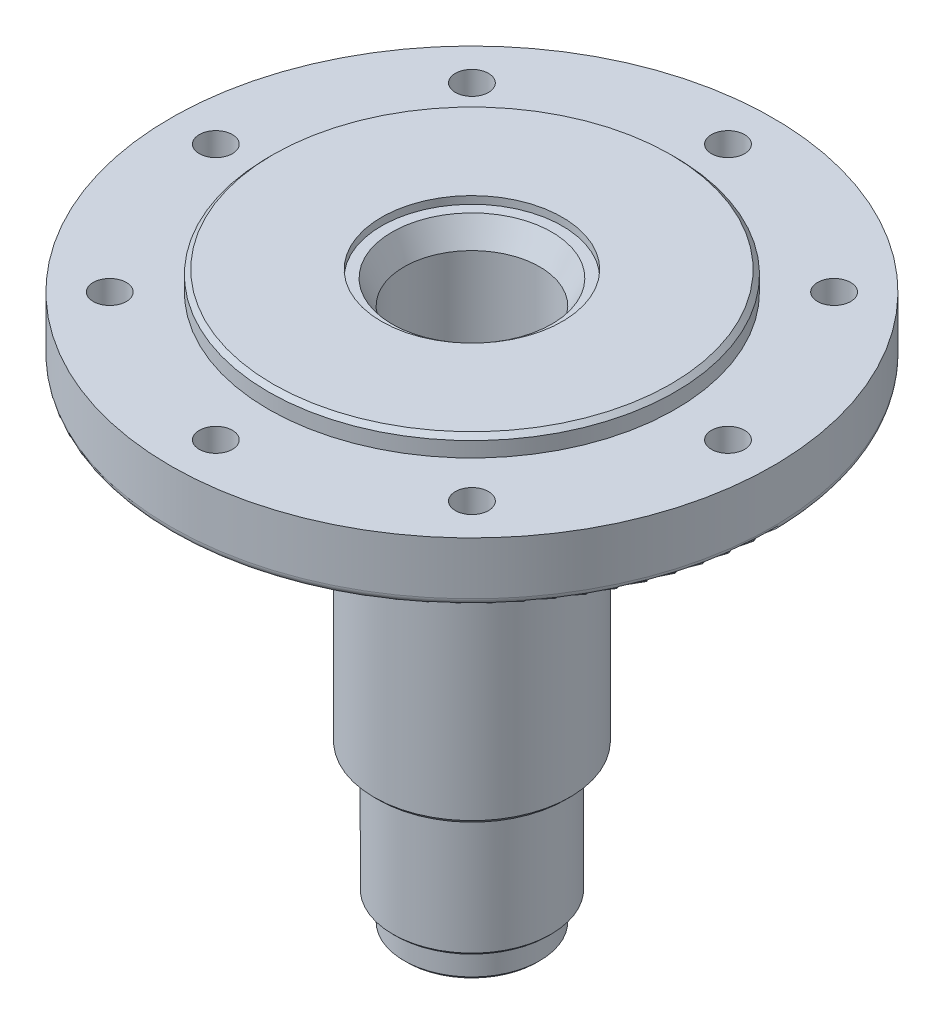
from build123d import *

# Parameters (mm, degrees)
SKETCH_2_R          = 20
CUT_EXTRUDE_1_DEPTH = 5
CUT_EXTRUDE_2_REACH = 424.606
SKETCH_3_R          = 11
SKETCH_5_R          = 120
SKETCH_5_R_2        = 80
CUT_EXTRUDE_3_DEPTH = 8
EXTRUDE_START       = 26
SKETCH_6_R          = 52.5
SKETCH_6_R_2        = 45
EXTRUDE_1_DEPTH     = 26
SKETCH_7_R          = 45
SKETCH_7_R_2        = 30
EXTRUDE_2_DEPTH     = 10
CHAMFER_1_SIZE      = 2
CHAMFER_2_SIZE      = 2


with BuildPart() as part:
    # 草图1 → 旋转1 (revolve)
    with BuildSketch(Plane.XY, mode=Mode.PRIVATE) as revolve_1_sk:
        with BuildLine():
            Line((60, 198.020625577), (132, 198.020625577))
            Line((132, 198.020625577), (135, 195.020625577))
            Line((135, 195.020625577), (135, 185.020625577))
            Line((135, 185.020625577), (200, 185.020625577))
            Line((200, 185.020625577), (200, 150.020625577))
            ThreePointArc((200, 150.020625577), (198.535533906, 146.485091671), (195, 145.020625577))
            Line((195, 145.020625577), (145, 145.020625577))
            Line((145, 145.020625577), (145, 140.020625577))
            Line((145, 140.020625577), (80, 140.020625577))
            Line((80, 140.020625577), (80, 87.020625577))
            Line((80, 87.020625577), (77, 84.020625577))
            Line((77, 84.020625577), (65, 84.020625577))
            Line((65, 84.020625577), (65, -72.979374423))
            Line((65, -72.979374423), (62, -75.979374423))
            Line((62, -75.979374423), (52.5, -75.979374423))
            Line((52.5, -75.979374423), (52.5, -131.979374423))
            Line((52.5, -131.979374423), (52.5, -133.979374423))
            Line((52.5, -133.979374423), (50.5, -133.979374423))
            Line((50.5, -133.979374423), (45, -133.979374423))
            Line((45, -133.979374423), (45, -167.979374423))
            Line((45, -167.979374423), (45, -168.979374423))
            Line((45, -168.979374423), (44, -168.979374423))
            Line((44, -168.979374423), (30, -168.979374423))
            Line((30, -168.979374423), (30, -36.979374423))
            Line((30, -36.979374423), (45, -20.479374423))
            Line((45, -20.479374423), (45, 177.020625577))
            Line((45, 177.020625577), (53, 193.020625577))
            Line((53, 193.020625577), (60, 193.020625577))
            Line((60, 193.020625577), (60, 198.020625577))
        make_face()
    revolve(revolve_1_sk.sketch.rotate(Axis((0, 246.142362889, 0), (0, -1, 0)), 90), axis=Axis((0, 246.142362889, 0), (0, -1, 0)))

    # 草图2 → 切除-拉伸1 (cut)
    with BuildSketch(Plane.XZ.offset(-145.020625577)):
        with Locations(Location((-120.208152802, 120.208152802, 0), (0, 0, 270))):
            Circle(SKETCH_2_R)
        with Locations(Location((-170, 0, 0), (0, 0, 270))):
            Circle(SKETCH_2_R)
        with Locations(Location((0, 170, 0), (0, 0, 270))):
            Circle(SKETCH_2_R)
        with Locations(Location((120.208152802, 120.208152802, 0), (0, 0, 270))):
            Circle(SKETCH_2_R)
        with Locations(Location((170, 0, 0), (0, 0, 270))):
            Circle(SKETCH_2_R)
        with Locations(Location((120.208152802, -120.208152802, 0), (0, 0, 270))):
            Circle(SKETCH_2_R)
        with Locations(Location((0, -170, 0), (0, 0, 270))):
            Circle(SKETCH_2_R)
        with Locations(Location((-120.208152802, -120.208152802, 0), (0, 0, 270))):
            Circle(SKETCH_2_R)
    extrude(amount=-CUT_EXTRUDE_1_DEPTH, mode=Mode.SUBTRACT)

    # 草图3 → 切除-拉伸2 (cut, up to next)
    with BuildSketch(Plane.XZ.offset(-145.020625577), mode=Mode.PRIVATE) as cut_extrude_2_sk1:
        with Locations(Location((-170, 0, 0), (0, 0, 270))):
            Circle(SKETCH_3_R)
    cut_extrude_2_tool1 = extrude(cut_extrude_2_sk1.sketch, amount=-CUT_EXTRUDE_2_REACH, mode=Mode.PRIVATE) & part.part
    # 草图3 → 切除-拉伸2 (cut, up to next)
    with BuildSketch(Plane.XZ.offset(-145.020625577), mode=Mode.PRIVATE) as cut_extrude_2_sk2:
        with Locations(Location((-120.208152802, 120.208152802, 0), (0, 0, 270))):
            Circle(SKETCH_3_R)
    cut_extrude_2_tool2 = extrude(cut_extrude_2_sk2.sketch, amount=-CUT_EXTRUDE_2_REACH, mode=Mode.PRIVATE) & part.part
    # 草图3 → 切除-拉伸2 (cut, up to next)
    with BuildSketch(Plane.XZ.offset(-145.020625577), mode=Mode.PRIVATE) as cut_extrude_2_sk3:
        with Locations(Location((0, 170, 0), (0, 0, 270))):
            Circle(SKETCH_3_R)
    cut_extrude_2_tool3 = extrude(cut_extrude_2_sk3.sketch, amount=-CUT_EXTRUDE_2_REACH, mode=Mode.PRIVATE) & part.part
    # 草图3 → 切除-拉伸2 (cut, up to next)
    with BuildSketch(Plane.XZ.offset(-145.020625577), mode=Mode.PRIVATE) as cut_extrude_2_sk4:
        with Locations(Location((120.208152802, 120.208152802, 0), (0, 0, 270))):
            Circle(SKETCH_3_R)
    cut_extrude_2_tool4 = extrude(cut_extrude_2_sk4.sketch, amount=-CUT_EXTRUDE_2_REACH, mode=Mode.PRIVATE) & part.part
    # 草图3 → 切除-拉伸2 (cut, up to next)
    with BuildSketch(Plane.XZ.offset(-145.020625577), mode=Mode.PRIVATE) as cut_extrude_2_sk5:
        with Locations(Location((170, 0, 0), (0, 0, 270))):
            Circle(SKETCH_3_R)
    cut_extrude_2_tool5 = extrude(cut_extrude_2_sk5.sketch, amount=-CUT_EXTRUDE_2_REACH, mode=Mode.PRIVATE) & part.part
    # 草图3 → 切除-拉伸2 (cut, up to next)
    with BuildSketch(Plane.XZ.offset(-145.020625577), mode=Mode.PRIVATE) as cut_extrude_2_sk6:
        with Locations(Location((120.208152802, -120.208152802, 0), (0, 0, 270))):
            Circle(SKETCH_3_R)
    cut_extrude_2_tool6 = extrude(cut_extrude_2_sk6.sketch, amount=-CUT_EXTRUDE_2_REACH, mode=Mode.PRIVATE) & part.part
    # 草图3 → 切除-拉伸2 (cut, up to next)
    with BuildSketch(Plane.XZ.offset(-145.020625577), mode=Mode.PRIVATE) as cut_extrude_2_sk7:
        with Locations(Location((0, -170, 0), (0, 0, 270))):
            Circle(SKETCH_3_R)
    cut_extrude_2_tool7 = extrude(cut_extrude_2_sk7.sketch, amount=-CUT_EXTRUDE_2_REACH, mode=Mode.PRIVATE) & part.part
    # 草图3 → 切除-拉伸2 (cut, up to next)
    with BuildSketch(Plane.XZ.offset(-145.020625577), mode=Mode.PRIVATE) as cut_extrude_2_sk8:
        with Locations(Location((-120.208152802, -120.208152802, 0), (0, 0, 270))):
            Circle(SKETCH_3_R)
    cut_extrude_2_tool8 = extrude(cut_extrude_2_sk8.sketch, amount=-CUT_EXTRUDE_2_REACH, mode=Mode.PRIVATE) & part.part
    add(cut_extrude_2_tool1.solids().sort_by_distance((-170, 145.020626, 0))[0], mode=Mode.SUBTRACT)
    add(cut_extrude_2_tool2.solids().sort_by_distance((-120.208153, 145.020626, 120.208153))[0], mode=Mode.SUBTRACT)
    add(cut_extrude_2_tool3.solids().sort_by_distance((0, 145.020626, 170))[0], mode=Mode.SUBTRACT)
    add(cut_extrude_2_tool4.solids().sort_by_distance((120.208153, 145.020626, 120.208153))[0], mode=Mode.SUBTRACT)
    add(cut_extrude_2_tool5.solids().sort_by_distance((170, 145.020626, 0))[0], mode=Mode.SUBTRACT)
    add(cut_extrude_2_tool6.solids().sort_by_distance((120.208153, 145.020626, -120.208153))[0], mode=Mode.SUBTRACT)
    add(cut_extrude_2_tool7.solids().sort_by_distance((0, 145.020626, -170))[0], mode=Mode.SUBTRACT)
    add(cut_extrude_2_tool8.solids().sort_by_distance((-120.208153, 145.020626, -120.208153))[0], mode=Mode.SUBTRACT)

    # 草图5 → 切除-拉伸3 (cut)
    with BuildSketch(Plane.XZ.offset(-140.020625577)):
        with Locations(Location((0, 0, 0), (0, 0, 270))):
            Circle(SKETCH_5_R)
        with Locations(Location((0, 0, 0), (0, 0, 90))):
            Circle(SKETCH_5_R_2, mode=Mode.SUBTRACT)
    extrude(amount=-CUT_EXTRUDE_3_DEPTH, mode=Mode.SUBTRACT)

    # 草图6 → 凸台-拉伸1 (add)
    with BuildSketch(Plane.XZ.offset(133.979374423).offset(EXTRUDE_START)):
        with Locations(Location((0, 0, 0), (0, 0, 90))):
            Circle(SKETCH_6_R)
        with Locations(Location((0, 0, 0), (0, 0, 90))):
            Circle(SKETCH_6_R_2, mode=Mode.SUBTRACT)
    extrude(amount=-EXTRUDE_1_DEPTH)

    # 草图7 → 凸台-拉伸2 (add)
    with BuildSketch(Plane.XZ.offset(168.979374423)):
        with Locations(Location((0, 0, 0), (0, 0, 90))):
            Circle(SKETCH_7_R)
        with Locations(Location((0, 0, 0), (0, 0, 90))):
            Circle(SKETCH_7_R_2, mode=Mode.SUBTRACT)
    extrude(amount=EXTRUDE_2_DEPTH)

    # 倒角1
    chamfer_1_edges = [part.edges().sort_by_distance(p)[0] for p in [
        (0, -159.979374423, -52.5),
    ]]
    chamfer(chamfer_1_edges, length=CHAMFER_1_SIZE)

    # 倒角2
    chamfer_2_edges = [part.edges().sort_by_distance(p)[0] for p in [
        (0, -178.979374423, -45),
    ]]
    chamfer(chamfer_2_edges, length=CHAMFER_2_SIZE)


solid = part.part
